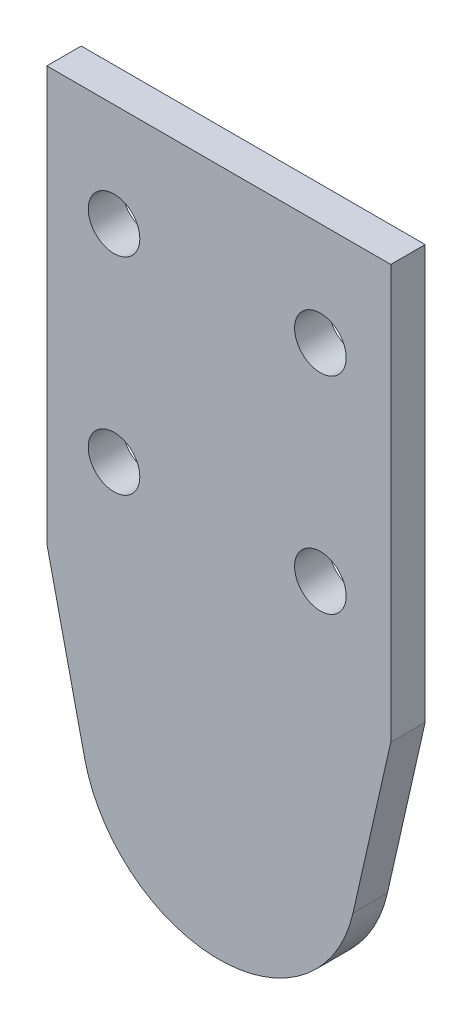
from build123d import *

# Parameters (mm, degrees)
SKETCH_1_R          = 20
EXTRUDE_1_DEPTH     = 10
CUT_EXTRUDE_1_DEPTH = 10
EXTRUDE_START       = -10
EXTRUDE_4_DEPTH     = 10
EXTRUDE_8_DEPTH     = 10
SKETCH_5_R          = 22.505017269
EXTRUDE_9_DEPTH     = 10


with BuildPart() as part:
    # 草图1 → 凸台-拉伸1 (new body)
    with BuildSketch(Plane.XY):
        with BuildLine():
            Line((0, 0), (90, 0))
            Line((90, 0), (84.980633901, -161.244553285))
            ThreePointArc((84.980633901, -161.244553285), (45, -200), (5.019366099, -161.244553285))
            Line((5.019366099, -161.244553285), (0, 0))
        make_face()
        with Locations((45, -160)):
            Circle(SKETCH_1_R, mode=Mode.SUBTRACT)
    extrude(amount=EXTRUDE_1_DEPTH)

    # 草图2 → 切除-拉伸1 (cut)
    with BuildSketch(Plane.XY.offset(10)):
        with BuildLine():
            Line((7.033066451, -30), (14.533066451, -30))
            Line((14.533066451, -30), (22.033066451, -30))
            ThreePointArc((22.033066451, -30), (14.533066451, -22.5), (7.033066451, -30))
        make_face()
        with BuildLine():
            Line((22.033066451, -30), (14.533066451, -30))
            Line((14.533066451, -30), (14.533066451, -37.5))
            ThreePointArc((14.533066451, -37.5), (19.83636731, -35.303300859), (22.033066451, -30))
        make_face()
        with BuildLine():
            Line((14.533066451, -37.5), (14.533066451, -30))
            Line((14.533066451, -30), (7.033066451, -30))
            ThreePointArc((7.033066451, -30), (9.229765592, -35.303300859), (14.533066451, -37.5))
        make_face()
        with BuildLine():
            Line((67.033066451, -30), (74.533066451, -30))
            Line((74.533066451, -30), (82.033066451, -30))
            ThreePointArc((82.033066451, -30), (74.533066451, -22.5), (67.033066451, -30))
        make_face()
        with BuildLine():
            ThreePointArc((67.033066451, -30), (69.229765592, -35.303300859), (74.533066451, -37.5))
            Line((74.533066451, -37.5), (74.533066451, -30))
            Line((74.533066451, -30), (67.033066451, -30))
        make_face()
        with BuildLine():
            Line((74.533066451, -30), (74.533066451, -37.5))
            ThreePointArc((74.533066451, -37.5), (79.83636731, -35.303300859), (82.033066451, -30))
            Line((82.033066451, -30), (74.533066451, -30))
        make_face()
        with BuildLine():
            ThreePointArc((74.533066451, -82.5), (69.229765592, -84.696699141), (67.033066451, -90))
            Line((67.033066451, -90), (74.533066451, -90))
            Line((74.533066451, -90), (74.533066451, -82.5))
        make_face()
        with BuildLine():
            Line((74.533066451, -90), (67.033066451, -90))
            ThreePointArc((67.033066451, -90), (74.533066451, -97.5), (82.033066451, -90))
            ThreePointArc((82.033066451, -90), (79.83636731, -84.696699141), (74.533066451, -82.5))
            Line((74.533066451, -82.5), (74.533066451, -90))
        make_face()
        with BuildLine():
            ThreePointArc((22.033066451, -90), (19.83636731, -84.696699141), (14.533066451, -82.5))
            Line((14.533066451, -82.5), (14.533066451, -90))
            Line((14.533066451, -90), (22.033066451, -90))
        make_face()
        with BuildLine():
            Line((14.533066451, -90), (14.533066451, -82.5))
            ThreePointArc((14.533066451, -82.5), (9.229765592, -95.303300859), (22.033066451, -90))
            Line((22.033066451, -90), (14.533066451, -90))
        make_face()
    extrude(amount=-CUT_EXTRUDE_1_DEPTH, mode=Mode.SUBTRACT)

    # 草图3 → 凸台-拉伸4 (add)
    with BuildSketch(Plane.XY.offset(10).offset(EXTRUDE_START)):
        with BuildLine():
            Line((5.019366099, -161.244553285), (0, 0))
            Line((0, 0), (0, -120))
            Line((0, -120), (5.275862069, -164.689655172))
            ThreePointArc((5.275862069, -164.689655172), (5.110404302, -162.969874585), (5.019366099, -161.244553285))
        make_face()
        with BuildLine():
            Line((90, 0), (84.980633901, -161.244553285))
            ThreePointArc((84.980633901, -161.244553285), (84.889595698, -162.969874585), (84.724137931, -164.689655172))
            Line((84.724137931, -164.689655172), (90, -120))
            Line((90, -120), (90, 0))
        make_face()
    extrude(amount=EXTRUDE_4_DEPTH)

    # 草图4 → 凸台-拉伸8 (add)
    with BuildSketch(Plane(origin=(0, 0, 0), x_dir=(-1, 0, 0), z_dir=(0, 0, -1))):
        with BuildLine():
            Line((-90, -120), (-90, 0))
            Line((-90, 0), (-95, 0))
            Line((-95, 0), (-95, -120.294117647))
            Line((-95, -120.294117647), (-84.012960099, -168.831134939))
            ThreePointArc((-84.012960099, -168.831134939), (-84.422970654, -166.769740378), (-84.724137931, -164.689655172))
            Line((-84.724137931, -164.689655172), (-90, -120))
        make_face()
        with BuildLine():
            Line((5, 0), (0, 0))
            Line((0, 0), (0, -120))
            Line((0, -120), (-5.275862069, -164.689655172))
            ThreePointArc((-5.275862069, -164.689655172), (-5.577029346, -166.769740378), (-5.987039901, -168.831134939))
            Line((-5.987039901, -168.831134939), (5, -120.294117647))
            Line((5, -120.294117647), (5, 0))
        make_face()
    extrude(amount=-EXTRUDE_8_DEPTH)

    # 草图5 → 凸台-拉伸9 (add)
    with BuildSketch(Plane(origin=(0, 0, 0), x_dir=(-1, 0, 0), z_dir=(0, 0, -1))):
        with Locations((-45, -160)):
            Circle(SKETCH_5_R)
    extrude(amount=-EXTRUDE_9_DEPTH)


solid = part.part
